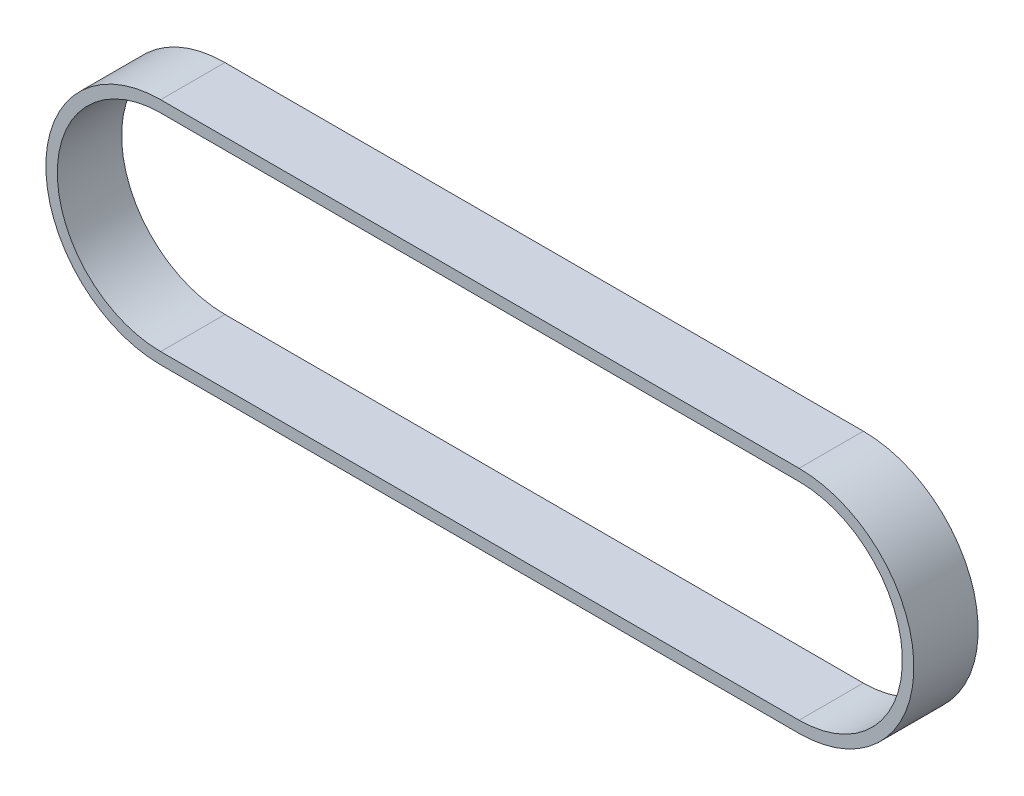
from build123d import *

# Parameters (mm, degrees)
EXTRUDE_1_DEPTH = 28


with BuildPart() as part:
    # 草图1 → 凸台-拉伸1 (new body)
    with BuildSketch(Plane.XY):
        with BuildLine():
            Line((0, 50), (278, 50))
            ThreePointArc((278, 50), (328, 0), (278, -50))
            Line((278, -50), (0, -50))
            ThreePointArc((0, -50), (-50, 0), (0, 50))
        make_face()
        with BuildLine():
            Line((0, 45), (278, 45))
            ThreePointArc((278, 45), (323, 0), (278, -45))
            Line((278, -45), (0, -45))
            ThreePointArc((0, -45), (-45, 0), (0, 45))
        make_face(mode=Mode.SUBTRACT)
    extrude(amount=EXTRUDE_1_DEPTH)


solid = part.part
